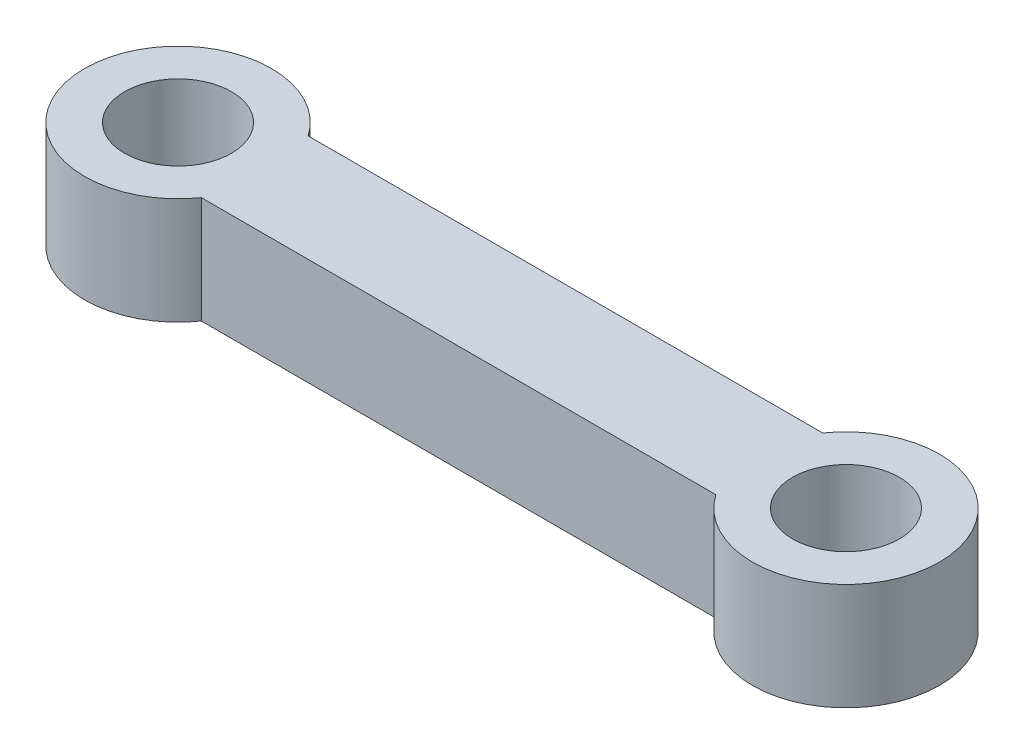
SolidWorks part; units mm, degrees
material "1060 Alloy"
ref_plane "Front Plane" through (0, 0, 0) normal (0, 0, 1) x (1, 0, 0)
ref_plane "Top Plane" through (0, 0, 0) normal (0, 1, 0) x (1, 0, 0)
ref_plane "Right Plane" through (0, 0, 0) normal (1, 0, 0) x (0, 0, -1)
sketch "Sketch1" plane through (0, 0, 0) normal (0, 1, 0) x (1, 0, 0)
  line L1 (5.7446, 4) -> (44.2554, 4)
  line L3 (5.7446, -4) -> (44.2554, -4)
  circle A0 centre (0, 0) radius 4
  arc A1 (5.7446, 4) -> (5.7446, -4) centre (0, 0) ccw
  circle A2 centre (50, 0) radius 4
  arc A3 (44.2554, -4) -> (44.2554, 4) centre (50, 0) ccw
  dimension "D1" = 8
  dimension "D2" = 8
  dimension "D3" = 14
  dimension "D4" = 14
  dimension "D5" = 50
extrude "Boss-Extrude1" add sketch "Sketch1" along normal blind 8
scale "Scale1" scale about origin uniform scaling yes scale factor 0.5
